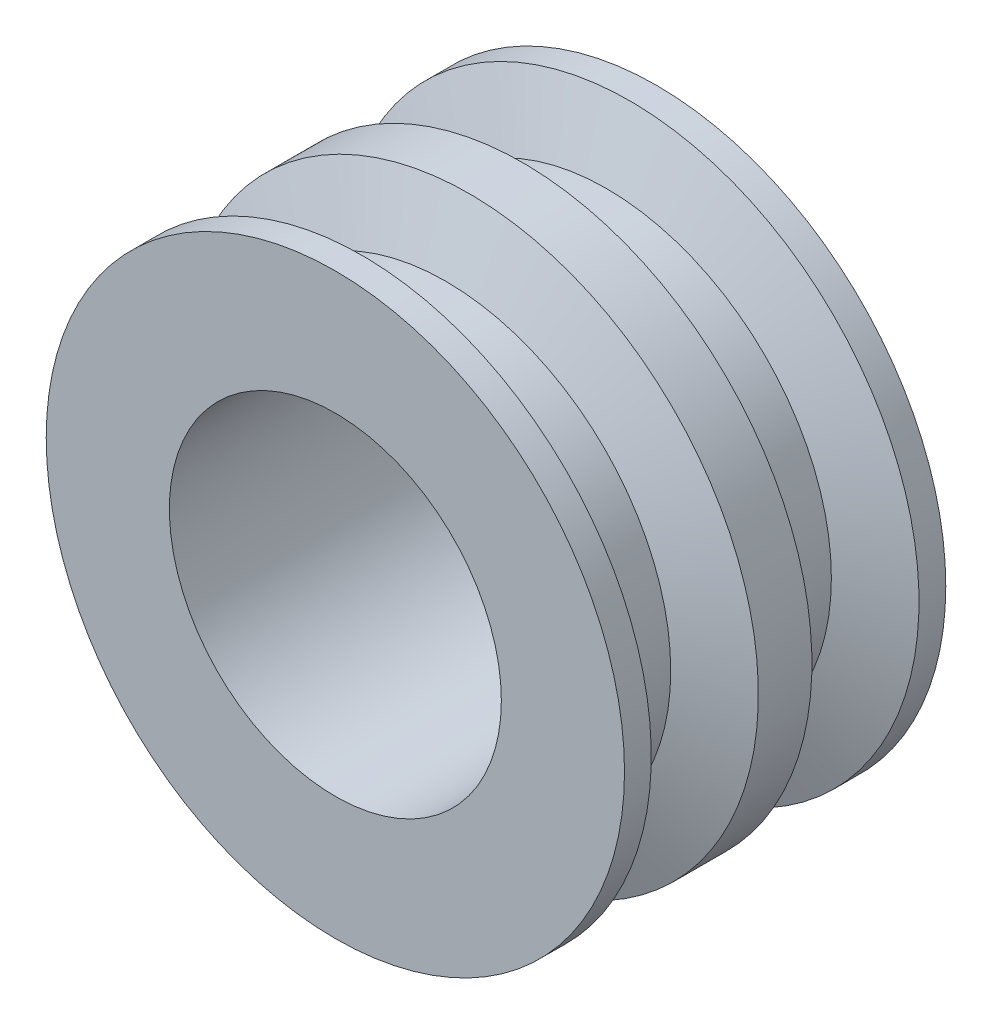
SolidWorks part; units mm, degrees
ref_plane "Front Plane" through (0, 0, 0) normal (0, 0, 1) x (1, 0, 0)
ref_plane "Top Plane" through (0, 0, 0) normal (0, 1, 0) x (1, 0, 0)
ref_plane "Right Plane" through (0, 0, 0) normal (1, 0, 0) x (0, 0, -1)
other "Configuration Table"
sketch "Sketch1" plane through (0, 0, 0) normal (0, 0, 1) x (1, 0, 0)
  circle A0 centre (0, 0) radius 27
  circle A1 centre (0, 0) radius 15.5
  dimension "D1" = 54
  dimension "D2" = 31
extrude "Boss-Extrude1" add sketch "Sketch1" along normal mid plane 30
sketch "Sketch2" plane through (0, 0, 0) normal (0, 1, 0) x (1, 0, 0)
  line L0 (-29.8563, 0) -> (27.1421, 0) construction
  line L2 (-27, 15) -> (-27, -15) construction
  line L6 (0, 19.2187) -> (0, -16.3425) construction
  line L9 (-30.1486, -7.5) -> (-13.3622, -7.5) construction
  line L11 (-27, -2.5) -> (-27, -12.5)
  line L12 (-27, -12.5) -> (-21, -10.3162)
  line L13 (-21, -4.6838) -> (-21, -10.3162)
  line L14 (-27, -2.5) -> (-21, -4.6838)
  line L15 (-30.1486, 7.5) -> (-13.3622, 7.5) construction
  line L16 (-27, 2.5) -> (-21, 4.6838)
  line L17 (-21, 4.6838) -> (-21, 10.3162)
  line L18 (-27, 12.5) -> (-21, 10.3162)
  line L19 (-27, 2.5) -> (-27, 12.5)
  point P11 (-27, 0)
  point P16 (-21, -7.5)
  point P17 (-27, -7.5)
  point P22 (-27, 7.5)
  point P23 (-21, 7.5)
  dimension "D1" = 7.5
  dimension "D2" = 10
  dimension "D3" = 40
  dimension "D4" = 6
revolve "Cut-Revolve1" cut sketch "Sketch2" angle 360 about L6
